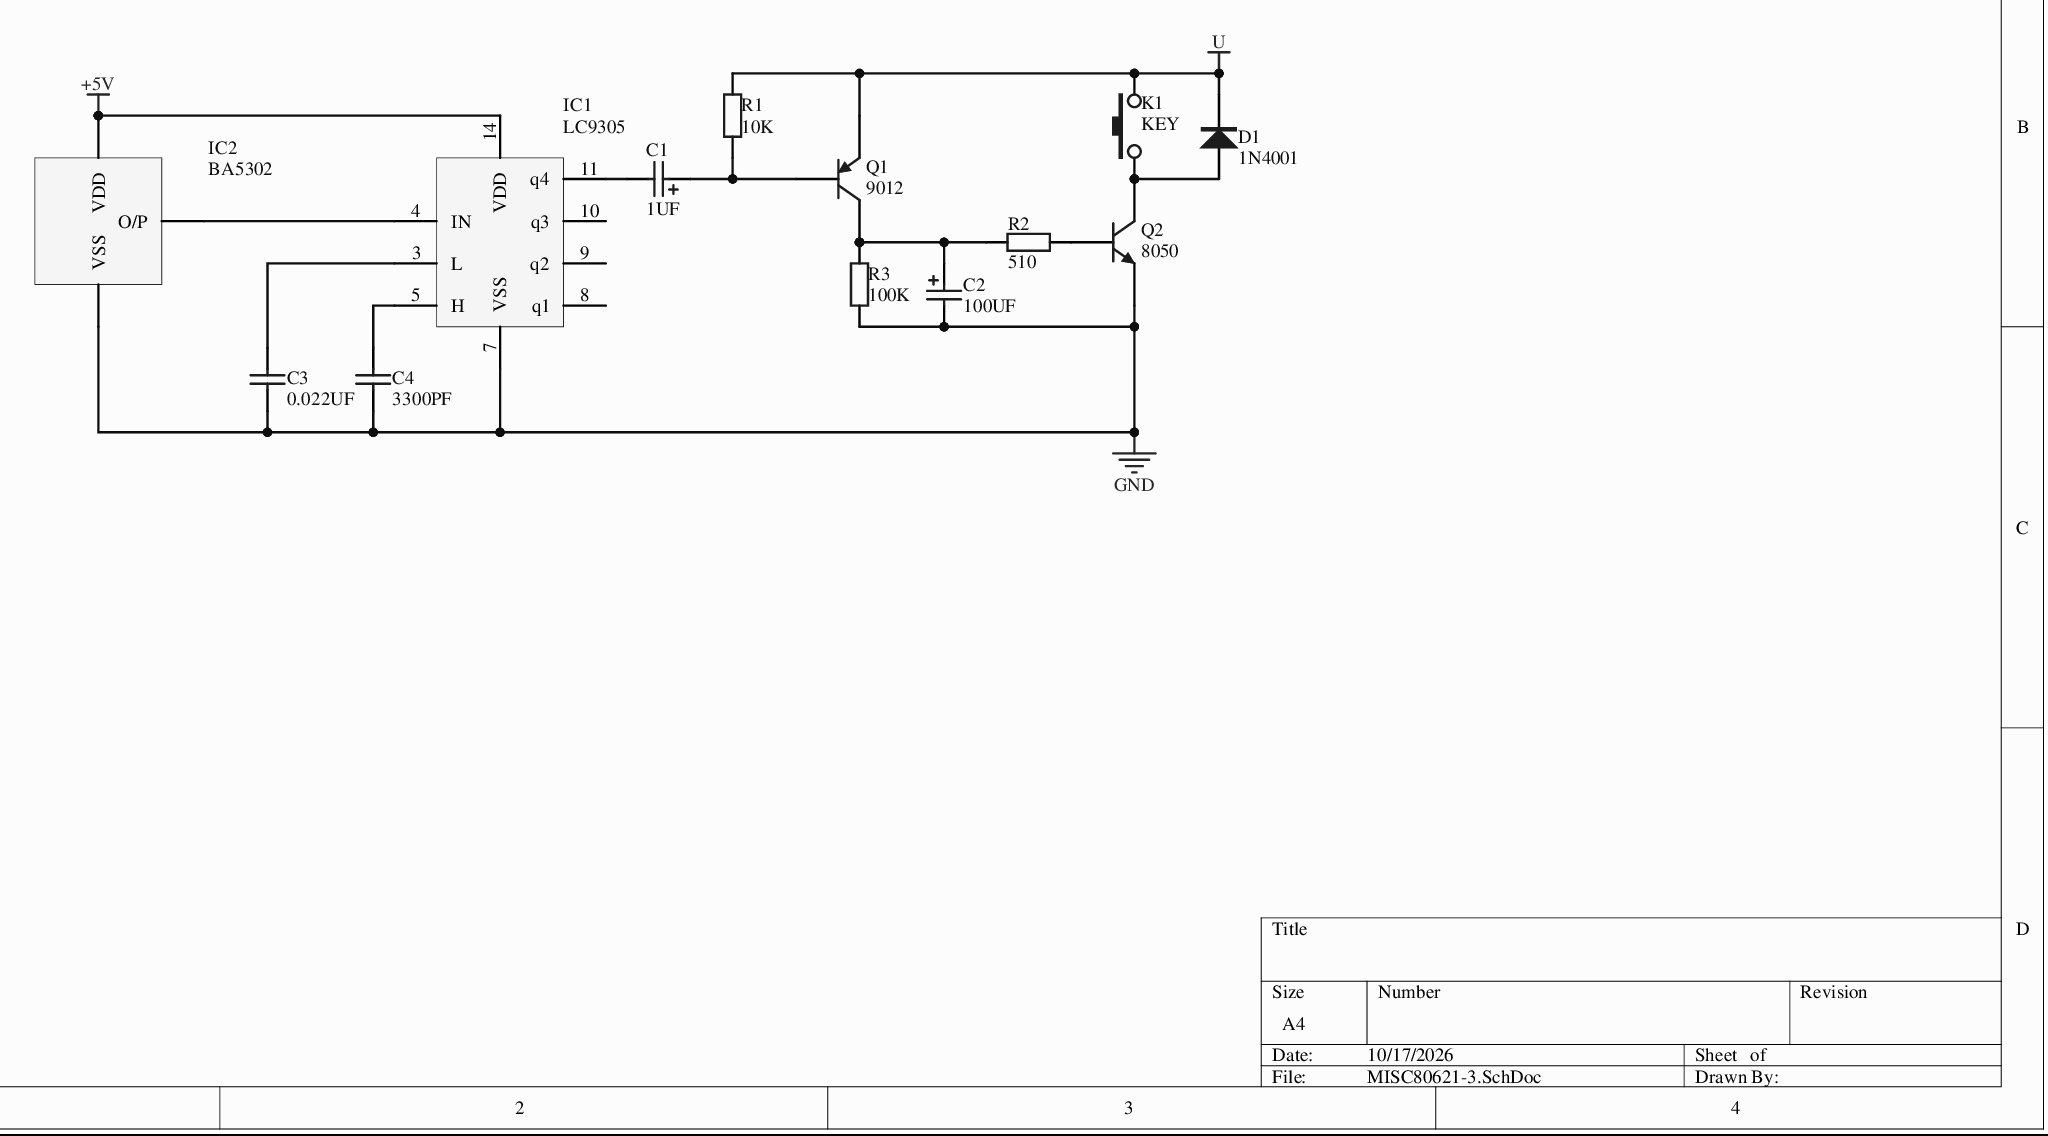
[diagram p0: MISC80621-3.SchDoc]
# Altium project MISC80621-6.PrjPcb
1 sheet, 13 parts. Net scope: global (net labels, ports and power ports of the same name join across sheets).
Board file: MISC80621.PcbDoc

## Sheet MISC80621-3.SchDoc
size A4

### Parts
C1  1UF  [POLAR0.8]
C2  100UF  [POLAR0.8]
C3  0.022UF  [RAD-0.3]
C4  3300PF  [RAD-0.3]
D1  1N4001  [DO-41]
IC1  LC9305  [DIP14]
IC2  BA5302  [HDR1X3]
K1  KEY  [DIP-3X6X4.3]
Q1  9012  [TO-92A]
Q2  8050  [TO-92A]
R1  10K  [AXIAL-0.4]
R2  510  [AXIAL-0.4]
R3  100K  [AXIAL-0.4]

### Nets
+5V: IC1.14(VDD) IC2.1(VDD)
GND: C2.2 C3.1 C4.1 IC1.7(VSS) IC2.3(VSS) Q2.1(E) R3.1
U: D1.2(K) K1.3 Q1.1(E) R1.2
NetC1_1: C1.1 Q1.2(B) R1.1
NetC1_2: C1.2 IC1.11(q4)
NetC2_1: C2.1 Q1.3(C) R2.2 R3.2
NetC3_2: C3.2 IC1.3(L)
NetC4_2: C4.2 IC1.5(H)
NetD1_1: D1.1(A) K1.1 Q2.3(C)
NetIC1_4: IC1.4(IN) IC2.2(O/P)
NetQ2_2: Q2.2(B) R2.1

Not connected (* = marked no-connect by the designer): IC1 8(q1) 9(q2) 10(q3)

### Library data of the parts
C1 C2 = Cap Pol2: Polarized Capacitor (Axial); Value: 100pF; Published: 8-Jun-2000; LatestRevisionDate: 17-Jul-2002; LatestRevisionNote: Re-released for DXP Platform.; PackageReference: POLAR0.8; PackageDescription: Polarized Capacitor; 2 Leads; Publisher: Altium Limited
C3 C4 = Cap: Capacitor; Value: 100pF; Published: 8-Jun-2000; LatestRevisionDate: 17-Jul-2002; LatestRevisionNote: Re-released for DXP Platform.; PackageReference: RAD-0.3; PackageDescription: Radial Cap, Thru-Hole; 2 Leads; 0.3 in Pin Spacing; Publisher: Altium Limited
D1 = 1N4007: Rectifier diode; BOM名称: Rectifier diode
Q1 = 2N3906: PNP General Purpose Amplifier; Published: 8-Jun-2000; LatestRevisionDate: 15-Jan-2003; LatestRevisionNote: PCB Footprint 'BCY-W3/D4.7' replaced; DatasheetVersion: 1997; PackageVersion: Sep-1998; PackageReference: TO-92A; PackageDescription: TO, Flat Index; 3 In-Line, Axial Leads; Body Dia. 4.5mm; Leads 0.51 x 0.48 mm (max); ComponentLink1Description: Manufacturer Link; ComponentLink2Description: Datasheet; ComponentLink2URL: http://example.com/ds/2N%2F2N3906.pdf; Publisher: Altium Limited
Q2 = 2N3904: NPN General Purpose Amplifier; Published: 8-Jun-2000; LatestRevisionDate: 15-Jan-2003; LatestRevisionNote: PCB Footprint 'BCY-W3/D4.7' replaced; DatasheetVersion: 1997; PackageVersion: Sep-1998; PackageReference: TO-92A; PackageDescription: TO, Flat Index; 3 In-Line, Axial Leads; Body Dia. 4.5mm; Leads 0.51 x 0.48 mm (max); ComponentLink1Description: Manufacturer Link; ComponentLink2Description: Datasheet; ComponentLink2URL: http://example.com/ds/2N%2F2N3904.pdf; Publisher: Altium Limited
R1-R3 = Res2: Resistor; Value: 1K; Published: 8-Jun-2000; LatestRevisionDate: 17-Jul-2002; LatestRevisionNote: Re-released for DXP Platform.; PackageReference: AXIAL-0.4; PackageDescription: Axial Device, Thru-Hole; 2 Leads; 0.4 in Pin Spacing; Publisher: Altium Limited